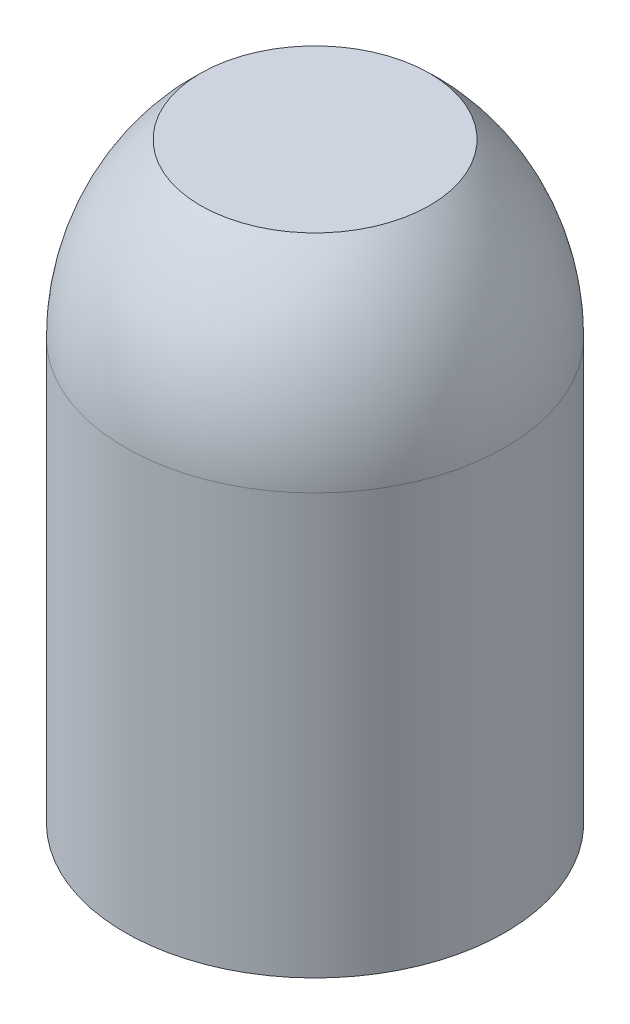
SolidWorks part; units mm, degrees
material "SUS304"
ref_plane "Front" through (0, 0, 0) normal (0, 0, 1) x (1, 0, 0)
ref_plane "Top" through (0, 0, 0) normal (0, 1, 0) x (1, 0, 0)
ref_plane "Right" through (0, 0, 0) normal (1, 0, 0) x (0, 0, -1)
sketch "Sketch1" plane through (0, 0, 0) normal (0, 0, 1) x (1, 0, 0)
  line L0 (0, 0) -> (0, 34.6592) construction
  line L1 (0, 0) -> (-4.975, 0)
  line L2 (-4.975, 0) -> (-4.975, 11)
  line L3 (-3, 15.5) -> (0, 15.5)
  line L4 (0, 15.5) -> (0, 0)
  arc A0 (-4.975, 11) -> (-3, 15.5) centre (1.1391, 11) cw
  dimension "D1" = 9.95
  dimension "D2" = 11
  dimension "D3" = 4.5
  dimension "D4" = 6
revolve "Revolve1" add sketch "Sketch1" angle 360 about L0
hole_wizard "M3 Tapped Hole1" positions "Sketch2" profile "Sketch3" tap size "M3" standard "GB"
sketch "Sketch2" plane through (0, 0, 0) normal (0, -1, 0) x (-1, 0, 0)
  point P0 (0, 0)
sketch "Sketch3" plane through (0, 0, 0) normal (1, 0, 0) x (0, 0, -1)
  line L0 (0, 0) -> (0, 8.2511)
  line L1 (0, 8.2511) -> (1.25, 7.5)
  line L2 (1.25, 7.5) -> (1.25, 0)
  line L5 (1.25, 0) -> (0, 0)
  line L10 (0, 8.2511) -> (-1.25, 7.5) construction
  line L11 (0, -6.35) -> (0, 107.95) construction
  dimension "螺纹孔钻头直径" = 2.5
  dimension "螺纹孔钻头深度" = 7.5
  dimension "导头角度" = 118
cosmetic thread "Cosmetic Thread1" parameters "D1"=6, "D2"=3
